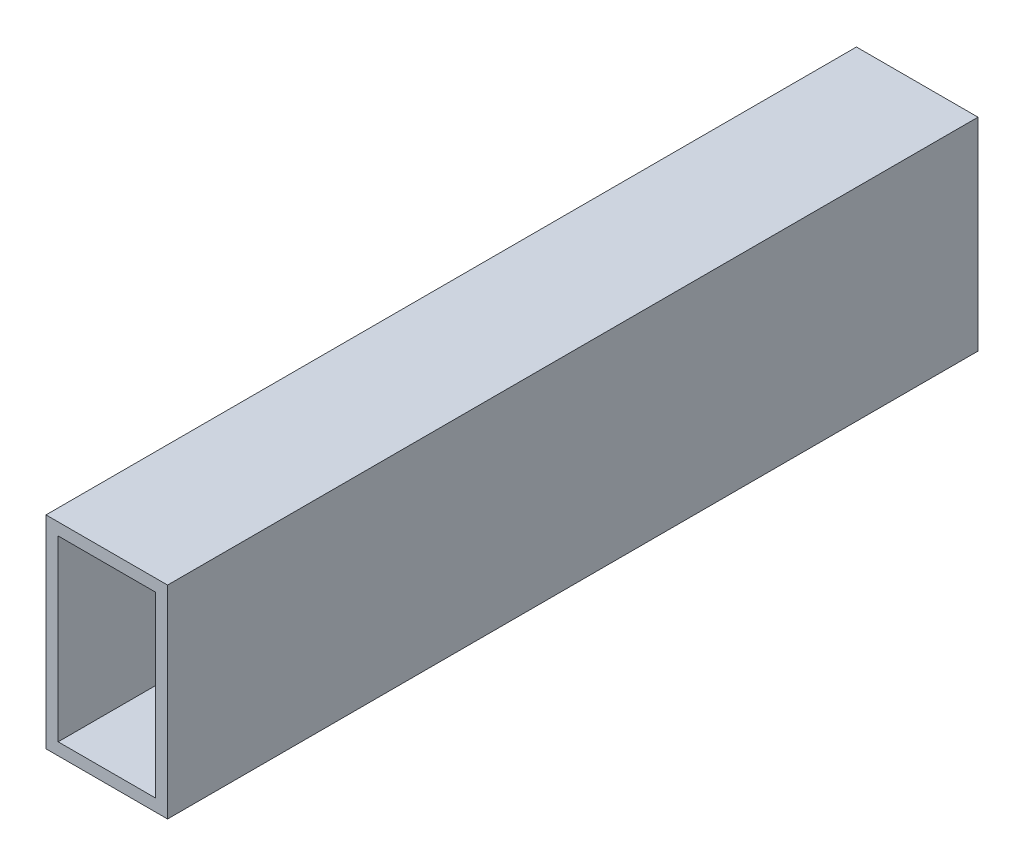
SolidWorks part; units mm, degrees
ref_plane "前视基准面" through (0, 0, 0) normal (0, 0, 1) x (1, 0, 0)
ref_plane "上视基准面" through (0, 0, 0) normal (0, 1, 0) x (1, 0, 0)
ref_plane "右视基准面" through (0, 0, 0) normal (1, 0, 0) x (0, 0, -1)
other "Configuration Table"
sketch "草图1" plane through (0, 0, 0) normal (0, 0, 1) x (1, 0, 0)
  line L0 (-15, -25) -> (15, -25)
  line L1 (15, -25) -> (15, 25)
  line L2 (15, 25) -> (-15, 25)
  line L3 (-15, 25) -> (-15, -25)
  line L4 (-12, -22) -> (12, -22)
  line L5 (12, -22) -> (12, 22)
  line L6 (12, 22) -> (-12, 22)
  line L7 (-12, 22) -> (-12, -22)
  point P0 (0, 0)
  dimension "D1" = 3
  dimension "D2" = 15
  dimension "D3" = 27
  dimension "D4" = 30
  dimension "D5" = 3
  dimension "D6" = 25
  dimension "D7" = 47
  dimension "D8" = 50
extrude "凸台-拉伸1" add sketch "草图1" against normal mid plane 200
